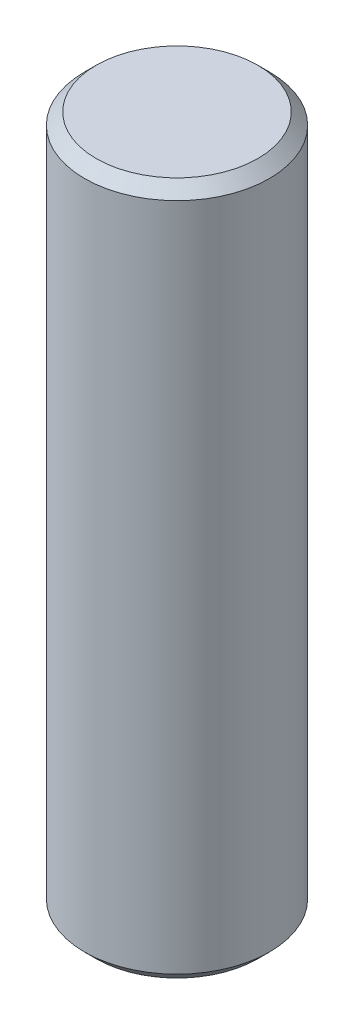
from build123d import *

# Parameters (mm, degrees)
SKETCH1_R           = 4
BOSS_EXTRUDE1_DEPTH = 15
CHAMFER1_SIZE       = 0.5


with BuildPart() as part:
    # Sketch1 → Boss-Extrude1 (new, symmetric)
    with BuildSketch(Plane(origin=(0, 0, 0), x_dir=(1, 0, 0), z_dir=(0, 1, 0))):
        with Locations(Location((0, 0, 0), (0, 0, 270))):
            Circle(SKETCH1_R)
    extrude(amount=BOSS_EXTRUDE1_DEPTH, both=True)

    # Chamfer1
    chamfer1_edges = [part.edges().sort_by_distance(p)[0] for p in [
        (0, -15, -4),
        (0, 15, -4),
    ]]
    chamfer(chamfer1_edges, length=CHAMFER1_SIZE)


solid = part.part
